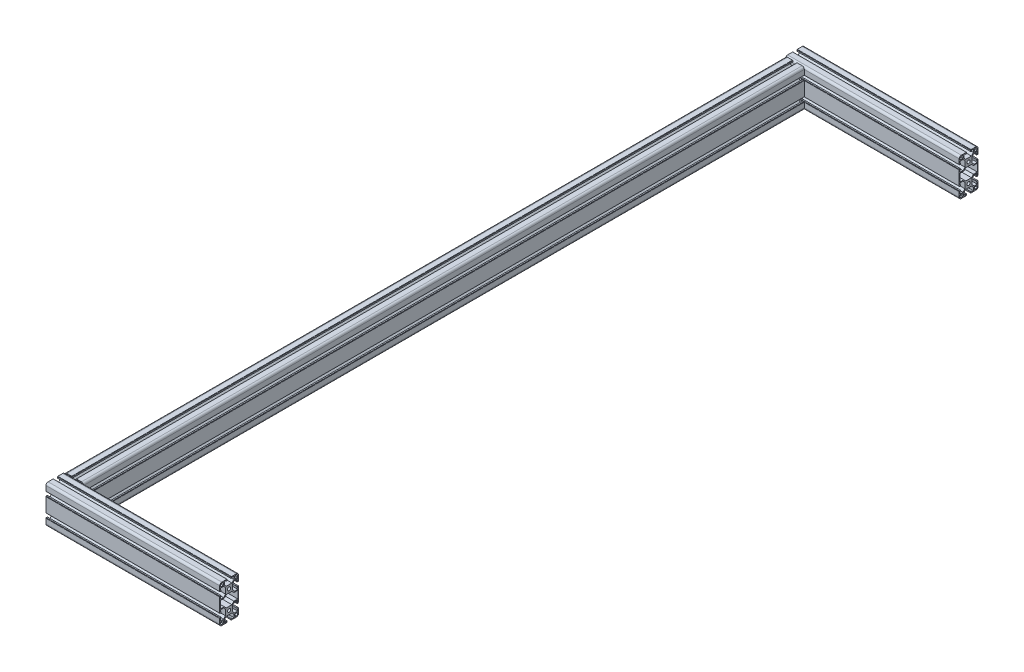
SolidWorks part; units mm, degrees
material "铝型材"
ref_plane "前基準面" through (0, 0, 0) normal (0, 0, 1) x (1, 0, 0)
ref_plane "上基準面" through (0, 0, 0) normal (0, 1, 0) x (1, 0, 0)
ref_plane "右基準面" through (0, 0, 0) normal (1, 0, 0) x (0, 0, -1)
sketch "草图1" plane through (0, 0, 0) normal (0, 1, 0) x (1, 0, 0)
  line L0 (0, -787.5) -> (0, 787.5)
  line L5 (0, -787.5) -> (350, -787.5)
  line L6 (350, -787.5) -> (350, 787.5)
  line L7 (350, 787.5) -> (0, 787.5)
  dimension "D1" = 1575
  dimension "D2" = 350
other "铝型材 40 X 80W X R4.5(1)"
ref_plane "基准面1" through (0, 0, 787.5) normal (0, 0, -1) x (-1, 0, 0)
sketch "Sketch1" plane through (0, 0, 787.5) normal (0, 0, -1) x (-1, 0, 0)
  line L0 (-5.1, 20) -> (-5.1, 19.5)
  line L1 (-5.1, 19.5) -> (-4.1, 19.5)
  line L2 (-4.1, 19.5) -> (-4.1, 17)
  line L3 (-6.1, 18.5) -> (-10.3, 18.5)
  line L4 (0, -20) -> (30.9704, -20) construction
  line L5 (-20, -34.775) -> (-20, -5.1)
  line L6 (15.5, 20) -> (5.1, 20)
  line L7 (20, 15.5) -> (20, 5.1)
  line L8 (0, 14.8756) -> (0, 0) construction
  line L9 (0, 0) -> (14.1675, 0) construction
  line L10 (-10.3, 18.5) -> (-10.3, 12)
  line L11 (-10.3, 12) -> (-6, 7.7)
  line L12 (-6, 7.7) -> (6, 7.7)
  line L13 (10.3, 12) -> (6, 7.7)
  line L14 (10.3, 18.5) -> (10.3, 12)
  line L15 (6.1, 18.5) -> (10.3, 18.5)
  line L16 (4.1, 19.5) -> (4.1, 17)
  line L17 (5.1, 19.5) -> (4.1, 19.5)
  line L18 (5.1, 20) -> (5.1, 19.5)
  line L19 (-5.1, 20) -> (-15.5, 20)
  line L20 (20, 5.1) -> (19.5, 5.1)
  line L21 (12.3, 18) -> (15.5, 18)
  line L22 (12.3, 18) -> (12.3, 12.3)
  line L23 (12.3, 12.3) -> (18, 12.3)
  line L24 (18, 15.5) -> (18, 12.3)
  line L25 (19.5, 5.1) -> (19.5, 4.1)
  line L26 (19.5, 4.1) -> (17, 4.1)
  line L27 (17, 6.1) -> (17, 4.1)
  line L28 (18.5, 6.1) -> (17, 6.1)
  line L29 (18.5, 6.1) -> (18.5, 10.3)
  line L30 (18.5, 10.3) -> (12, 10.3)
  line L31 (12, 10.3) -> (7.7, 6)
  line L32 (7.7, 6) -> (7.7, -6)
  line L33 (12, -10.3) -> (7.7, -6)
  line L34 (18.5, -10.3) -> (12, -10.3)
  line L35 (18.5, -6.1) -> (18.5, -10.3)
  line L36 (18.5, -6.1) -> (17, -6.1)
  line L37 (17, -4.1) -> (17, -6.1)
  line L38 (19.5, -4.1) -> (17, -4.1)
  line L39 (19.5, -5.1) -> (19.5, -4.1)
  line L40 (20, -5.1) -> (19.5, -5.1)
  line L41 (5.1, 20) -> (-5.1, 20) construction
  line L42 (-5.1, -60) -> (5.1, -60) construction
  line L43 (0, 0) -> (20, 0) construction
  line L44 (20, 0) -> (40, 0) construction
  line L45 (0, 0) -> (-20, 0) construction
  line L46 (-20, 0) -> (-40, 0) construction
  line L47 (0, -40) -> (20, -40) construction
  line L48 (10.325, -12.025) -> (6, -7.7)
  line L49 (6, -7.7) -> (-6, -7.7)
  line L50 (-10.325, -12.025) -> (-6, -7.7)
  line L51 (20, -40) -> (40, -40) construction
  line L52 (0, -40) -> (-20, -40) construction
  line L53 (-20, -40) -> (-40, -40) construction
  line L58 (-20, -5.1) -> (-19.5, -5.1)
  line L60 (-20, 5.1) -> (-20, 15.5)
  line L61 (-19.5, -5.1) -> (-19.5, -4.1)
  line L62 (-6.1, 18.5) -> (-6.1, 17)
  line L63 (-6.1, 17) -> (-4.1, 17)
  line L64 (6.1, 18.5) -> (6.1, 17)
  line L65 (4.1, 17) -> (6.1, 17)
  line L66 (-19.5, -4.1) -> (-17, -4.1)
  line L67 (-15.5, 18) -> (-12.3, 18)
  line L68 (-18, 15.5) -> (-18, 12.3)
  line L69 (-18, 12.3) -> (-12.3, 12.3)
  line L70 (-12.3, 18) -> (-12.3, 12.3)
  line L71 (-17, -6.1) -> (-17, -4.1)
  line L72 (-18.5, -6.1) -> (-17, -6.1)
  line L73 (-18.5, -6.1) -> (-18.5, -10.3)
  line L74 (-18.5, -10.3) -> (-12, -10.3)
  line L75 (-12, -10.3) -> (-7.7, -6)
  line L76 (-7.7, -6) -> (-7.7, 6)
  line L77 (-12, 10.3) -> (-7.7, 6)
  line L78 (-18.5, 10.3) -> (-12, 10.3)
  line L79 (-18.5, 6.1) -> (-18.5, 10.3)
  line L80 (-18.5, 6.1) -> (-17, 6.1)
  line L81 (-17, 4.1) -> (-17, 6.1)
  line L82 (-19.5, 4.1) -> (-17, 4.1)
  line L83 (-19.5, 5.1) -> (-19.5, 4.1)
  line L84 (-20, 5.1) -> (-19.5, 5.1)
  line L85 (20, -5.1) -> (20, -34.9003)
  line L87 (-18.5, -12.025) -> (-10.325, -12.025)
  line L88 (-18.5, -12.025) -> (-18.5, -28)
  line L91 (10.325, -12.025) -> (18.5, -12.025)
  line L94 (18.5, -12.025) -> (18.5, -28)
  line L100 (10.3, -28) -> (18.5, -28)
  line L104 (-18.5, -28) -> (-10.3, -28)
  line L106 (-20, -44.975) -> (-19.5, -44.975)
  line L107 (-19.5, -44.975) -> (-19.5, -43.975)
  line L108 (-19.5, -43.975) -> (-17, -43.975)
  line L109 (-17, -43.975) -> (-17, -45.975)
  line L110 (-18.5, -45.975) -> (-17, -45.975)
  line L111 (-18.5, -45.975) -> (-18.5, -50.175)
  line L112 (-18.5, -50.175) -> (-12, -50.175)
  line L113 (-12, -50.175) -> (-7.7, -45.875)
  line L114 (-7.7, -33.875) -> (-7.7, -45.875)
  line L115 (-12, -29.575) -> (-7.7, -33.875)
  line L116 (-18.5, -29.575) -> (-12, -29.575)
  line L117 (-18.5, -33.775) -> (-18.5, -29.575)
  line L118 (-18.5, -33.775) -> (-17, -33.775)
  line L119 (-17, -33.775) -> (-17, -35.775)
  line L120 (-12.3017, -58) -> (-12.3017, -52.3)
  line L121 (-18.0017, -52.3) -> (-12.3017, -52.3)
  line L122 (-18.0017, -55.5) -> (-18.0017, -52.3)
  line L123 (-15.5017, -58) -> (-12.3017, -58)
  line L124 (-19.5, -35.775) -> (-17, -35.775)
  line L125 (4.1, -57) -> (6.1, -57)
  line L126 (6.1, -58.5) -> (6.1, -57)
  line L127 (-6.1, -57) -> (-4.1, -57)
  line L128 (-6.1, -58.5) -> (-6.1, -57)
  line L129 (-19.5, -34.775) -> (-19.5, -35.775)
  line L130 (-20, -44.975) -> (-20, -55.375)
  line L131 (-20, -34.775) -> (-19.5, -34.775)
  line L138 (-10.3, -28) -> (-6, -32.3)
  line L139 (6, -32.3) -> (-6, -32.3)
  line L140 (10.3, -28) -> (6, -32.3)
  line L147 (20, -34.9003) -> (19.375, -34.8976)
  line L148 (19.375, -34.8976) -> (19.3708, -35.8976)
  line L149 (19.3708, -35.8976) -> (16.8708, -35.8871)
  line L150 (16.8708, -35.8871) -> (16.8792, -33.8872)
  line L151 (18.3792, -33.8935) -> (16.8792, -33.8872)
  line L152 (18.3792, -33.8935) -> (18.3968, -29.6935)
  line L153 (18.3968, -29.6935) -> (11.8969, -29.6662)
  line L154 (11.8969, -29.6662) -> (7.5789, -33.9482)
  line L155 (7.5285, -45.948) -> (7.5789, -33.9482)
  line L156 (11.8105, -50.266) -> (7.5285, -45.948)
  line L157 (18.3104, -50.2933) -> (11.8105, -50.266)
  line L158 (18.328, -46.0933) -> (18.3104, -50.2933)
  line L159 (18.328, -46.0933) -> (16.828, -46.0871)
  line L160 (16.828, -46.0871) -> (16.8364, -44.0871)
  line L161 (19.3364, -44.0976) -> (16.8364, -44.0871)
  line L162 (19.3322, -45.0976) -> (19.3364, -44.0976)
  line L163 (18, -55.5) -> (18, -52.3)
  line L164 (12.3, -52.3) -> (18, -52.3)
  line L165 (12.3, -58) -> (12.3, -52.3)
  line L166 (12.3, -58) -> (15.5, -58)
  line L167 (20, -45.1004) -> (19.3322, -45.0976)
  line L168 (-5.1, -60) -> (-15.5017, -60)
  line L169 (5.1, -60) -> (5.1, -59.5)
  line L170 (5.1, -59.5) -> (4.1, -59.5)
  line L171 (4.1, -59.5) -> (4.1, -57)
  line L172 (6.1, -58.5) -> (10.3, -58.5)
  line L173 (10.3, -58.5) -> (10.3, -52)
  line L174 (10.3, -52) -> (6, -47.7)
  line L175 (-6, -47.7) -> (6, -47.7)
  line L176 (-10.3, -52) -> (-6, -47.7)
  line L177 (-10.3, -58.5) -> (-10.3, -52)
  line L178 (20, -55.5) -> (20, -45.1004)
  line L179 (15.5, -60) -> (5.1, -60)
  line L181 (-6.1, -58.5) -> (-10.3, -58.5)
  line L182 (-4.1, -59.5) -> (-4.1, -57)
  line L183 (-5.1, -59.5) -> (-4.1, -59.5)
  line L184 (-5.1, -60) -> (-5.1, -59.5)
  line L185 (5.1, -20) -> (5.1, -19.5) [skipped]
  line L186 (5.1, -19.5) -> (4.1, -19.5) [skipped]
  line L187 (4.1, -19.5) -> (4.1, -17) [skipped]
  line L188 (6.1, -17) -> (4.1, -17) [skipped]
  line L189 (6.1, -18.5) -> (6.1, -17) [skipped]
  line L190 (6.1, -18.5) -> (10.3, -18.5) [skipped]
  line L191 (-6.1, -18.5) -> (-10.3, -18.5) [skipped]
  line L192 (-6.1, -18.5) -> (-6.1, -17) [skipped]
  line L193 (-4.1, -17) -> (-6.1, -17) [skipped]
  line L194 (-4.1, -19.5) -> (-4.1, -17) [skipped]
  line L195 (-5.1, -19.5) -> (-4.1, -19.5) [skipped]
  line L196 (-5.1, -20) -> (-5.1, -19.5) [skipped]
  line L197 (-10.3, -18.5) -> (-10.3, -12) [skipped]
  line L198 (10.3, -18.5) -> (10.3, -12) [skipped]
  circle A0 centre (0, 0) radius 3.4
  arc A1 (-20, 15.5) -> (-15.5, 20) centre (-15.5, 15.5) cw
  arc A2 (20, 15.5) -> (15.5, 20) centre (15.5, 15.5) ccw
  arc A5 (-15.5, 18) -> (-18, 15.5) centre (-15.5, 15.5) ccw
  arc A6 (18, 15.5) -> (15.5, 18) centre (15.5, 15.5) ccw
  arc A11 (18, -55.5) -> (15.5, -58) centre (15.5, -55.5) cw
  arc A12 (-15.5017, -58) -> (-18.0017, -55.5) centre (-15.5017, -55.5) cw
  arc A15 (20, -55.5) -> (15.5, -60) centre (15.5, -55.5) cw
  arc A16 (-20, -55.375) -> (-15.5017, -60) centre (-15.5017, -55.5) ccw
  circle A17 centre (0, -40) radius 3.4
  point P2 (0, 10)
  point P4 (0, 0)
  point P7 (20, 20)
  point P8 (-20, 20)
  point P12 (-20, -20.0001)
  point P15 (20, -20.0001)
  point P36 (-20, 20)
  point P39 (20, 20)
  point P40 (0, 20)
  point P42 (0, -60)
  point P75 (0, 0)
  dimension "D1" = 20.6
  dimension "D2" = 40
  dimension "D3" = 8.2
  dimension "D4" = 10.2
  dimension "D5" = 12.3
  dimension "D6" = 6.8
  dimension "D7" = 4.5
  dimension "D8" = 45
  dimension "D12" = 2
  dimension "D13" = 5.7
  dimension "D14" = 2
  dimension "D18" = 2.5
  dimension "D19" = 2.5
  dimension "D15" = 80
  dimension "D9" = 0.5
  dimension "D10" = 1.5
  dimension "D11" = 12
  dimension "D16" = 3
  dimension "D17" = 2
  dimension "D20" = 2
  dimension "D21" = 20
  dimension "D22" = 1.725
  dimension "D23" = 20
other "铝型材 40 X 80W X R4.5(7)"
ref_plane "基准面2" through (0, 0, 787.5) normal (1, 0, 0) x (0, 0, -1)
sketch "Sketch11" plane through (0, 0, 787.5) normal (1, 0, 0) x (0, 0, -1)
  line L0 (-5.1, 20) -> (-5.1, 19.5)
  line L1 (-5.1, 19.5) -> (-4.1, 19.5)
  line L2 (-4.1, 19.5) -> (-4.1, 17)
  line L3 (-6.1, 18.5) -> (-10.3, 18.5)
  line L4 (0, -20) -> (30.9704, -20) construction
  line L5 (-20, -34.775) -> (-20, -5.1)
  line L6 (15.5, 20) -> (5.1, 20)
  line L7 (20, 15.5) -> (20, 5.1)
  line L8 (0, 14.8756) -> (0, 0) construction
  line L9 (0, 0) -> (14.1675, 0) construction
  line L10 (-10.3, 18.5) -> (-10.3, 12)
  line L11 (-10.3, 12) -> (-6, 7.7)
  line L12 (-6, 7.7) -> (6, 7.7)
  line L13 (10.3, 12) -> (6, 7.7)
  line L14 (10.3, 18.5) -> (10.3, 12)
  line L15 (6.1, 18.5) -> (10.3, 18.5)
  line L16 (4.1, 19.5) -> (4.1, 17)
  line L17 (5.1, 19.5) -> (4.1, 19.5)
  line L18 (5.1, 20) -> (5.1, 19.5)
  line L19 (-5.1, 20) -> (-15.5, 20)
  line L20 (20, 5.1) -> (19.5, 5.1)
  line L21 (12.3, 18) -> (15.5, 18)
  line L22 (12.3, 18) -> (12.3, 12.3)
  line L23 (12.3, 12.3) -> (18, 12.3)
  line L24 (18, 15.5) -> (18, 12.3)
  line L25 (19.5, 5.1) -> (19.5, 4.1)
  line L26 (19.5, 4.1) -> (17, 4.1)
  line L27 (17, 6.1) -> (17, 4.1)
  line L28 (18.5, 6.1) -> (17, 6.1)
  line L29 (18.5, 6.1) -> (18.5, 10.3)
  line L30 (18.5, 10.3) -> (12, 10.3)
  line L31 (12, 10.3) -> (7.7, 6)
  line L32 (7.7, 6) -> (7.7, -6)
  line L33 (12, -10.3) -> (7.7, -6)
  line L34 (18.5, -10.3) -> (12, -10.3)
  line L35 (18.5, -6.1) -> (18.5, -10.3)
  line L36 (18.5, -6.1) -> (17, -6.1)
  line L37 (17, -4.1) -> (17, -6.1)
  line L38 (19.5, -4.1) -> (17, -4.1)
  line L39 (19.5, -5.1) -> (19.5, -4.1)
  line L40 (20, -5.1) -> (19.5, -5.1)
  line L41 (5.1, 20) -> (-5.1, 20) construction
  line L42 (-5.1, -60) -> (5.1, -60) construction
  line L43 (0, 0) -> (20, 0) construction
  line L44 (20, 0) -> (40, 0) construction
  line L45 (0, 0) -> (-20, 0) construction
  line L46 (-20, 0) -> (-40, 0) construction
  line L47 (0, -40) -> (20, -40) construction
  line L48 (10.325, -12.025) -> (6, -7.7)
  line L49 (6, -7.7) -> (-6, -7.7)
  line L50 (-10.325, -12.025) -> (-6, -7.7)
  line L51 (20, -40) -> (40, -40) construction
  line L52 (0, -40) -> (-20, -40) construction
  line L53 (-20, -40) -> (-40, -40) construction
  line L58 (-20, -5.1) -> (-19.5, -5.1)
  line L60 (-20, 5.1) -> (-20, 15.5)
  line L61 (-19.5, -5.1) -> (-19.5, -4.1)
  line L62 (-6.1, 18.5) -> (-6.1, 17)
  line L63 (-6.1, 17) -> (-4.1, 17)
  line L64 (6.1, 18.5) -> (6.1, 17)
  line L65 (4.1, 17) -> (6.1, 17)
  line L66 (-19.5, -4.1) -> (-17, -4.1)
  line L67 (-15.5, 18) -> (-12.3, 18)
  line L68 (-18, 15.5) -> (-18, 12.3)
  line L69 (-18, 12.3) -> (-12.3, 12.3)
  line L70 (-12.3, 18) -> (-12.3, 12.3)
  line L71 (-17, -6.1) -> (-17, -4.1)
  line L72 (-18.5, -6.1) -> (-17, -6.1)
  line L73 (-18.5, -6.1) -> (-18.5, -10.3)
  line L74 (-18.5, -10.3) -> (-12, -10.3)
  line L75 (-12, -10.3) -> (-7.7, -6)
  line L76 (-7.7, -6) -> (-7.7, 6)
  line L77 (-12, 10.3) -> (-7.7, 6)
  line L78 (-18.5, 10.3) -> (-12, 10.3)
  line L79 (-18.5, 6.1) -> (-18.5, 10.3)
  line L80 (-18.5, 6.1) -> (-17, 6.1)
  line L81 (-17, 4.1) -> (-17, 6.1)
  line L82 (-19.5, 4.1) -> (-17, 4.1)
  line L83 (-19.5, 5.1) -> (-19.5, 4.1)
  line L84 (-20, 5.1) -> (-19.5, 5.1)
  line L85 (20, -5.1) -> (20, -34.9003)
  line L87 (-18.5, -12.025) -> (-10.325, -12.025)
  line L88 (-18.5, -12.025) -> (-18.5, -28)
  line L91 (10.325, -12.025) -> (18.5, -12.025)
  line L94 (18.5, -12.025) -> (18.5, -28)
  line L100 (10.3, -28) -> (18.5, -28)
  line L104 (-18.5, -28) -> (-10.3, -28)
  line L106 (-20, -44.975) -> (-19.5, -44.975)
  line L107 (-19.5, -44.975) -> (-19.5, -43.975)
  line L108 (-19.5, -43.975) -> (-17, -43.975)
  line L109 (-17, -43.975) -> (-17, -45.975)
  line L110 (-18.5, -45.975) -> (-17, -45.975)
  line L111 (-18.5, -45.975) -> (-18.5, -50.175)
  line L112 (-18.5, -50.175) -> (-12, -50.175)
  line L113 (-12, -50.175) -> (-7.7, -45.875)
  line L114 (-7.7, -33.875) -> (-7.7, -45.875)
  line L115 (-12, -29.575) -> (-7.7, -33.875)
  line L116 (-18.5, -29.575) -> (-12, -29.575)
  line L117 (-18.5, -33.775) -> (-18.5, -29.575)
  line L118 (-18.5, -33.775) -> (-17, -33.775)
  line L119 (-17, -33.775) -> (-17, -35.775)
  line L120 (-12.3017, -58) -> (-12.3017, -52.3)
  line L121 (-18.0017, -52.3) -> (-12.3017, -52.3)
  line L122 (-18.0017, -55.5) -> (-18.0017, -52.3)
  line L123 (-15.5017, -58) -> (-12.3017, -58)
  line L124 (-19.5, -35.775) -> (-17, -35.775)
  line L125 (4.1, -57) -> (6.1, -57)
  line L126 (6.1, -58.5) -> (6.1, -57)
  line L127 (-6.1, -57) -> (-4.1, -57)
  line L128 (-6.1, -58.5) -> (-6.1, -57)
  line L129 (-19.5, -34.775) -> (-19.5, -35.775)
  line L130 (-20, -44.975) -> (-20, -55.375)
  line L131 (-20, -34.775) -> (-19.5, -34.775)
  line L138 (-10.3, -28) -> (-6, -32.3)
  line L139 (6, -32.3) -> (-6, -32.3)
  line L140 (10.3, -28) -> (6, -32.3)
  line L147 (20, -34.9003) -> (19.375, -34.8976)
  line L148 (19.375, -34.8976) -> (19.3708, -35.8976)
  line L149 (19.3708, -35.8976) -> (16.8708, -35.8871)
  line L150 (16.8708, -35.8871) -> (16.8792, -33.8872)
  line L151 (18.3792, -33.8935) -> (16.8792, -33.8872)
  line L152 (18.3792, -33.8935) -> (18.3968, -29.6935)
  line L153 (18.3968, -29.6935) -> (11.8969, -29.6662)
  line L154 (11.8969, -29.6662) -> (7.5789, -33.9482)
  line L155 (7.5285, -45.948) -> (7.5789, -33.9482)
  line L156 (11.8105, -50.266) -> (7.5285, -45.948)
  line L157 (18.3104, -50.2933) -> (11.8105, -50.266)
  line L158 (18.328, -46.0933) -> (18.3104, -50.2933)
  line L159 (18.328, -46.0933) -> (16.828, -46.0871)
  line L160 (16.828, -46.0871) -> (16.8364, -44.0871)
  line L161 (19.3364, -44.0976) -> (16.8364, -44.0871)
  line L162 (19.3322, -45.0976) -> (19.3364, -44.0976)
  line L163 (18, -55.5) -> (18, -52.3)
  line L164 (12.3, -52.3) -> (18, -52.3)
  line L165 (12.3, -58) -> (12.3, -52.3)
  line L166 (12.3, -58) -> (15.5, -58)
  line L167 (20, -45.1004) -> (19.3322, -45.0976)
  line L168 (-5.1, -60) -> (-15.5017, -60)
  line L169 (5.1, -60) -> (5.1, -59.5)
  line L170 (5.1, -59.5) -> (4.1, -59.5)
  line L171 (4.1, -59.5) -> (4.1, -57)
  line L172 (6.1, -58.5) -> (10.3, -58.5)
  line L173 (10.3, -58.5) -> (10.3, -52)
  line L174 (10.3, -52) -> (6, -47.7)
  line L175 (-6, -47.7) -> (6, -47.7)
  line L176 (-10.3, -52) -> (-6, -47.7)
  line L177 (-10.3, -58.5) -> (-10.3, -52)
  line L178 (20, -55.5) -> (20, -45.1004)
  line L179 (15.5, -60) -> (5.1, -60)
  line L181 (-6.1, -58.5) -> (-10.3, -58.5)
  line L182 (-4.1, -59.5) -> (-4.1, -57)
  line L183 (-5.1, -59.5) -> (-4.1, -59.5)
  line L184 (-5.1, -60) -> (-5.1, -59.5)
  line L185 (5.1, -20) -> (5.1, -19.5) [skipped]
  line L186 (5.1, -19.5) -> (4.1, -19.5) [skipped]
  line L187 (4.1, -19.5) -> (4.1, -17) [skipped]
  line L188 (6.1, -17) -> (4.1, -17) [skipped]
  line L189 (6.1, -18.5) -> (6.1, -17) [skipped]
  line L190 (6.1, -18.5) -> (10.3, -18.5) [skipped]
  line L191 (-6.1, -18.5) -> (-10.3, -18.5) [skipped]
  line L192 (-6.1, -18.5) -> (-6.1, -17) [skipped]
  line L193 (-4.1, -17) -> (-6.1, -17) [skipped]
  line L194 (-4.1, -19.5) -> (-4.1, -17) [skipped]
  line L195 (-5.1, -19.5) -> (-4.1, -19.5) [skipped]
  line L196 (-5.1, -20) -> (-5.1, -19.5) [skipped]
  line L197 (-10.3, -18.5) -> (-10.3, -12) [skipped]
  line L198 (10.3, -18.5) -> (10.3, -12) [skipped]
  circle A0 centre (0, 0) radius 3.4
  arc A1 (-20, 15.5) -> (-15.5, 20) centre (-15.5, 15.5) cw
  arc A2 (20, 15.5) -> (15.5, 20) centre (15.5, 15.5) ccw
  arc A5 (-15.5, 18) -> (-18, 15.5) centre (-15.5, 15.5) ccw
  arc A6 (18, 15.5) -> (15.5, 18) centre (15.5, 15.5) ccw
  arc A11 (18, -55.5) -> (15.5, -58) centre (15.5, -55.5) cw
  arc A12 (-15.5017, -58) -> (-18.0017, -55.5) centre (-15.5017, -55.5) cw
  arc A15 (20, -55.5) -> (15.5, -60) centre (15.5, -55.5) cw
  arc A16 (-20, -55.375) -> (-15.5017, -60) centre (-15.5017, -55.5) ccw
  circle A17 centre (0, -40) radius 3.4
  point P2 (0, 10)
  point P4 (0, 0)
  point P7 (20, 20)
  point P8 (-20, 20)
  point P12 (-20, -20.0001)
  point P15 (20, -20.0001)
  point P36 (-20, 20)
  point P39 (20, 20)
  point P40 (0, 20)
  point P42 (0, -60)
  point P75 (0, 0)
  dimension "D1" = 20.6
  dimension "D2" = 40
  dimension "D3" = 8.2
  dimension "D4" = 10.2
  dimension "D5" = 12.3
  dimension "D6" = 6.8
  dimension "D7" = 4.5
  dimension "D8" = 45
  dimension "D12" = 2
  dimension "D13" = 5.7
  dimension "D14" = 2
  dimension "D18" = 2.5
  dimension "D19" = 2.5
  dimension "D15" = 80
  dimension "D9" = 0.5
  dimension "D10" = 1.5
  dimension "D11" = 12
  dimension "D16" = 3
  dimension "D17" = 2
  dimension "D20" = 2
  dimension "D21" = 20
  dimension "D22" = 1.725
  dimension "D23" = 20
other "剪裁/延伸2"
other "剪裁/延伸3"
